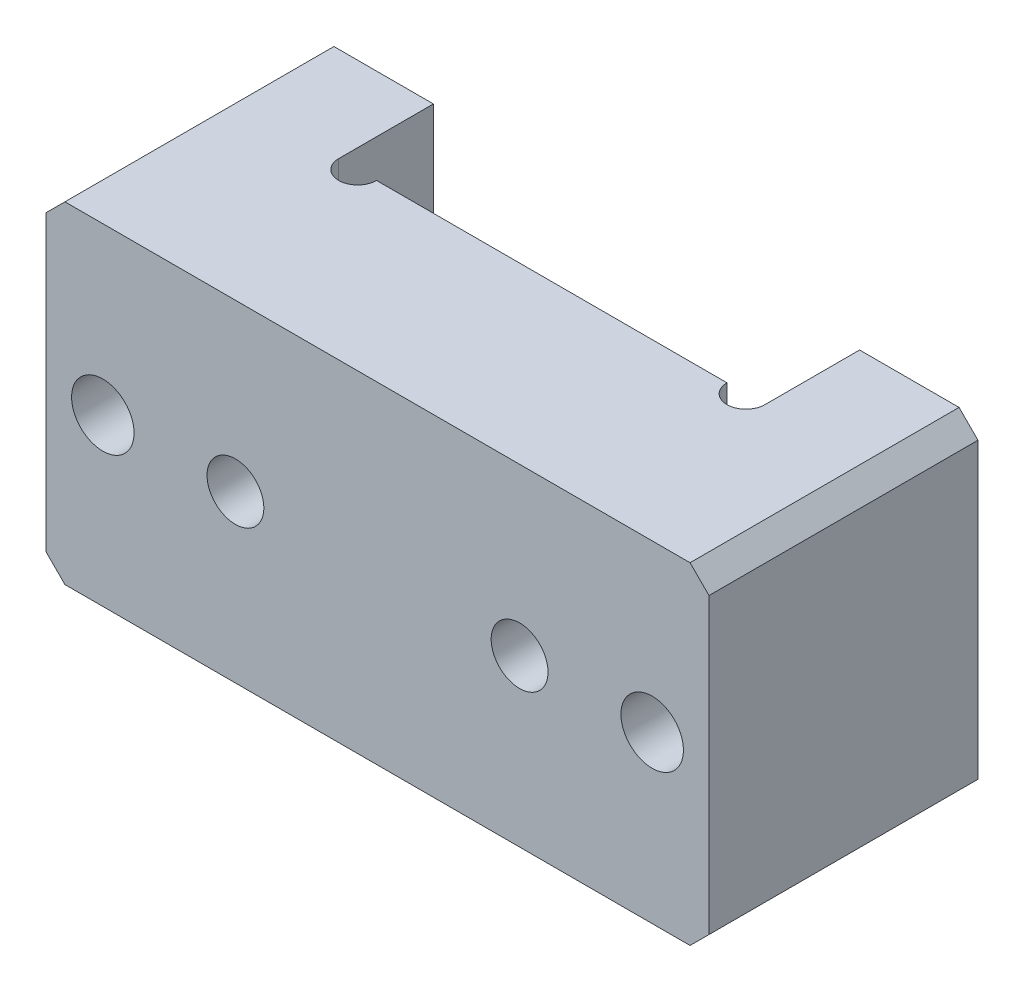
SolidWorks part; units mm, degrees
material "S45C"
ref_plane "前视基准面" through (0, 0, 0) normal (0, 0, 1) x (1, 0, 0)
ref_plane "上视基准面" through (0, 0, 0) normal (0, 1, 0) x (1, 0, 0)
ref_plane "右视基准面" through (0, 0, 0) normal (1, 0, 0) x (0, 0, -1)
sketch "草图1" plane through (0, 0, 0) normal (0, 1, 0) x (1, 0, 0)
  line L0 (-35, 0) -> (35, 0)
  line L1 (35, 0) -> (35, 28.4)
  line L2 (35, 28.4) -> (22.5, 28.4)
  line L3 (22.5, 28.4) -> (22.5, 18.4)
  line L4 (22.5, 18.4) -> (-22.5, 18.4)
  line L5 (-22.5, 18.4) -> (-22.5, 28.4)
  line L6 (-22.5, 28.4) -> (-35, 28.4)
  line L7 (-35, 28.4) -> (-35, 0)
  line L8 (0, 0) -> (0, 61.464) construction
  dimension "D1" = 45
  dimension "D2" = 10
  dimension "D3" = 18.4
  dimension "D4" = 70
extrude "凸台-拉伸1" add sketch "草图1" along normal mid plane 35
sketch "草图2" plane through (0, 17.5, 0) normal (0, 1, 0) x (1, 0, 0)
  line L0 (22.5, 18.4) -> (-22.5, 18.4) construction
  circle A1 centre (20.5, 18.4) radius 2
  circle A2 centre (-20.5, 18.4) radius 2
  dimension "D1" = 4
extrude "切除-拉伸1" cut sketch "草图2" against normal up to next
chamfer "倒角1" distance 2 angle 45 4 edges at (-35, -17.5, -14.2) (35, -17.5, -14.2) (35, 17.5, -14.2) (-35, 17.5, -14.2)
sketch "草图3" plane through (0, 0, 0) normal (0, 0, 1) x (1, 0, 0)
  line L0 (0, 17.5) -> (0, -22.0481) construction
  line L1 (-33, 17.5) -> (33, 17.5) construction
  point P0 (-15, 0)
  point P2 (15, 0)
  dimension "D1" = 30
hole_wizard "Ø6.0mm 暗销孔1" positions "草图3" profile "草图4" hole size "Ø6.0" standard "GB"
sketch "草图4" plane through (-15, 0, 0) normal (1, 0, 0) x (0, -1, 0)
  line L0 (0, 0) -> (0, 16.8026)
  line L1 (0, 16.8026) -> (3, 15)
  line L2 (3, 15) -> (3, 0)
  line L5 (3, 0) -> (0, 0)
  line L10 (0, 16.8026) -> (-3, 15) construction
  line L11 (0, -6.35) -> (0, 107.95) construction
  dimension "孔直径" = 6
  dimension "孔深度" = 15
  dimension "导头角度" = 118
sketch "草图5" plane through (0, 0, -28.4) normal (0, 0, -1) x (-1, 0, 0)
  line L0 (0, 0) -> (0, -28.8931) construction
  point P0 (-29, 0)
  point P2 (29, 0)
  dimension "D1" = 58
hole_wizard "M6 六角圆柱头螺钉的柱形沉头孔1" positions "草图5" profile "草图6" counterbore size "M6" standard "GB" end condition up to next
sketch "草图6" plane through (29, 0, -28.4) normal (1, 0, 0) x (0, 1, 0)
  line L0 (0, 0) -> (0, 28.4)
  line L1 (0, 28.4) -> (3.3, 28.4)
  line L3 (3.3, 28.4) -> (3.3, 6.8)
  line L4 (3.3, 6.8) -> (5.5, 6.8)
  line L5 (5.5, 6.8) -> (5.5, 0)
  line L7 (5.5, 0) -> (0, 0)
  line L11 (0, -6.35) -> (0, 107.95) construction
  dimension "通孔孔直径" = 6.6
  dimension "通孔孔深度" = 28.4
  dimension "柱形沉头孔直径" = 11
  dimension "柱形沉头孔深度" = 6.8
sketch "草图7" plane through (0, 0, -28.4) normal (0, 0, -1) x (-1, 0, 0)
  line L0 (0, 0) -> (41.1565, 0) construction
  line L3 (0, 0) -> (0, -22.251) construction
  point P0 (-29, 12.5)
  point P2 (-29, -12.5)
  point P4 (29, 12.5)
  point P6 (29, -12.5)
  dimension "D1" = 58
  dimension "D2" = 25
hole_wizard "M4 螺纹孔1" positions "草图7" profile "草图8" tap size "M4" standard "GB"
sketch "草图8" plane through (29, 12.5, -28.4) normal (1, 0, 0) x (0, 1, 0)
  line L0 (0, 0) -> (0, 19.4914)
  line L1 (0, 19.4914) -> (1.65, 18.5)
  line L2 (1.65, 18.5) -> (1.65, 0)
  line L5 (1.65, 0) -> (0, 0)
  line L10 (0, 19.4914) -> (-1.65, 18.5) construction
  line L11 (0, -6.35) -> (0, 107.95) construction
  dimension "螺纹孔钻头直径" = 3.3
  dimension "螺纹孔钻头深度" = 18.5
  dimension "导头角度" = 118
cosmetic thread "孔螺纹线1" parameters "D1"=15, "D2"=4
cosmetic thread "孔螺纹线2" parameters "D1"=15, "D2"=4
cosmetic thread "孔螺纹线3" parameters "D1"=15, "D2"=4
cosmetic thread "孔螺纹线4" parameters "D1"=15, "D2"=4
